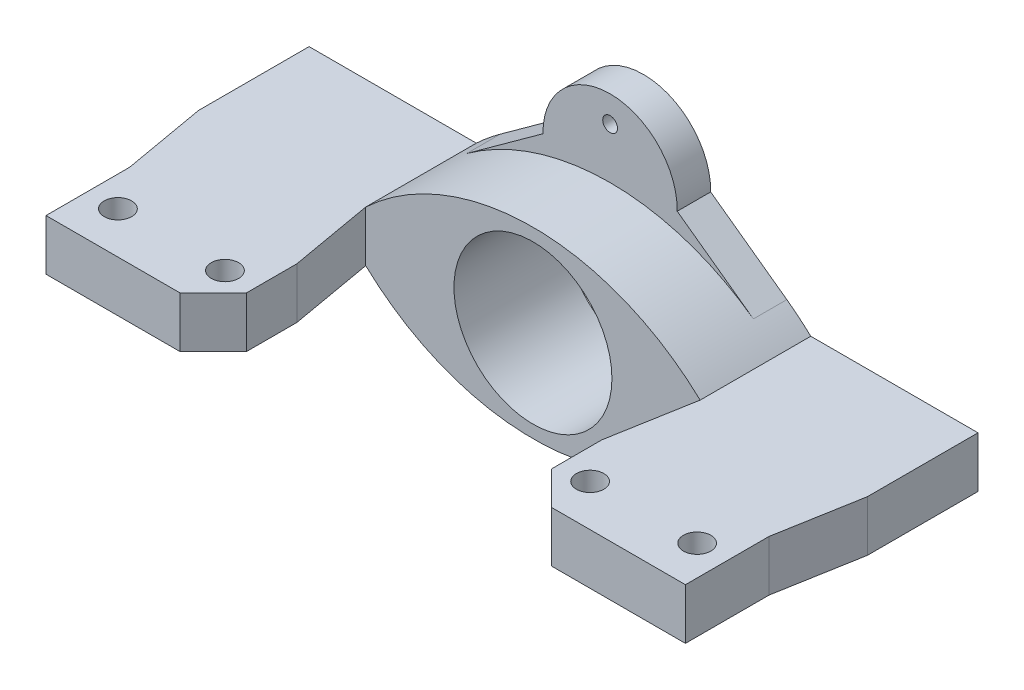
SolidWorks part; units mm, degrees
ref_plane "Front Plane" through (0, 0, 0) normal (0, 0, 1) x (1, 0, 0)
ref_plane "Top Plane" through (0, 0, 0) normal (0, 1, 0) x (1, 0, 0)
ref_plane "Right Plane" through (0, 0, 0) normal (1, 0, 0) x (0, 0, -1)
sketch "Sketch1" plane through (0, 0, 0) normal (0, 0, 1) x (1, 0, 0)
  line L1 (-25.7118, -19.05) -> (25.7118, -19.05)
  line L2 (-25.7118, -19.05) -> (-25.7118, 19.05)
  line L3 (-25.7118, 19.05) -> (25.7118, 19.05)
  line L4 (25.7118, -19.05) -> (25.7118, 19.05)
  line L5 (-25.7118, -19.05) -> (25.7118, 19.05) construction
  line L6 (-25.7118, 19.05) -> (25.7118, -19.05) construction
  line L7 (-63.5, -19.05) -> (63.5, -19.05)
  line L8 (-63.5, -19.05) -> (-63.5, 19.05)
  line L9 (-63.5, 19.05) -> (63.5, 19.05)
  line L10 (63.5, -19.05) -> (63.5, 19.05)
  line L11 (-63.5, -19.05) -> (63.5, 19.05) construction
  line L12 (-63.5, 19.05) -> (63.5, -19.05) construction
  circle A0 centre (0, 0) radius 15 construction
  circle A1 centre (0, 0) radius 15
  circle A2 centre (0, 0) radius 32 construction
  circle A3 centre (0, 0) radius 32
  dimension "D1" = 38.1
  dimension "D2" = 127
extrude "Boss-Extrude1" add sketch "Sketch1" against normal up to surface (21 mm away) contours A1 L3 L2 L1 | L2 A3 | A1 L1 L4 L3 | L4 A3 | A3 L9 L8 L7 | A3 L7 L10 L9
sketch "Sketch3" plane through (0, 0, -21) normal (0, 0, -1) x (-1, 0, 0)
  line L0 (0, 0) -> (0, -27) construction
  line L2 (-63.5, -19.05) -> (63.5, -19.05)
  line L3 (63.5, 19.05) -> (-63.5, 19.05)
  line L4 (-63.5, -19.05) -> (63.5, -19.05)
  line L5 (63.5, 19.05) -> (-63.5, 19.05)
  line L9 (63.5, -19.05) -> (63.5, 19.05)
  line L10 (63.5, -19.05) -> (63.5, 19.05)
  line L11 (-63.5, 19.05) -> (-63.5, -19.05)
  line L12 (-63.5, 19.05) -> (-63.5, -19.05)
  arc A0 (12.7437, -19.05) -> (-12.7437, -19.05) centre (0, -19.2546) cw
  circle A1 centre (0, 0) radius 32
  circle A6 centre (0, 0) radius 32
  dimension "D1" = 0
  dimension "D2" = 0
extrude "Boss-Extrude2" add sketch "Sketch3" against normal blind 6.35
sketch "Sketch4" plane through (0, 0, -14.65) normal (0, 0, 1) x (1, 0, 0)
  line L1 (12.7437, -19.05) -> (-12.7437, -19.05)
  line L2 (12.7437, -19.05) -> (-12.7437, -19.05)
  circle A0 centre (0, -27) radius 1.4 construction
  arc A1 (-12.7437, -19.05) -> (12.7437, -19.05) centre (0, -19.2546) ccw
  arc A2 (-12.7437, -19.05) -> (12.7437, -19.05) centre (0, -19.2546) ccw
  circle A3 centre (0, -27) radius 1.4
  dimension "D1" = 0
extrude "Cut-Extrude2" cut sketch "Sketch4" against normal blind 6.35 contours A3
ref_plane "Plane1" through (0, 0, 0) normal (0, 1, 0) x (1, 0, 0)
mirror "Mirror1" about plane through (0, 0, 0) normal (0, 1, 0) of "Boss-Extrude2", "Cut-Extrude2"
sketch "Sketch5" plane through (0, 0, 0) normal (0, 0, 1) x (1, 0, 0)
  line L0 (-63.5, 0) -> (0, 0) construction
  line L1 (-63.5, -4.826) -> (63.5, -4.826)
  line L2 (-63.5, -4.826) -> (-63.5, 4.826)
  line L3 (-63.5, 4.826) -> (63.5, 4.826)
  line L4 (-63.5, -19.05) -> (63.5, -19.05)
  line L5 (63.5, -19.05) -> (63.5, 19.05)
  line L6 (63.5, 19.05) -> (-63.5, 19.05)
  line L7 (-63.5, 19.05) -> (-63.5, -19.05)
  line L8 (-63.5, -19.05) -> (63.5, -19.05)
  line L9 (63.5, -19.05) -> (63.5, 19.05)
  line L10 (63.5, 19.05) -> (-63.5, 19.05)
  line L11 (-63.5, 19.05) -> (-63.5, -19.05)
  line L12 (63.5, -4.826) -> (63.5, 4.826)
  line L13 (-63.5, -4.826) -> (63.5, 4.826) construction
  line L14 (-63.5, 4.826) -> (63.5, -4.826) construction
  line L15 (0, 48.7566) -> (0, -50.4513) construction
  circle A0 centre (0, 0) radius 15 construction
  circle A1 centre (0, 0) radius 15
  arc A2 (31.75, 4.826) -> (-31.75, 4.826) centre (0, -28.9962) ccw
  arc A3 (31.75, -4.826) -> (-31.75, -4.826) centre (0, 28.9962) cw
  point P2 (0, 0)
  point P17 (-31.75, 0)
  circle M7 centre (0, 0) radius 15
  line M8 (-63.5, -19.05) -> (63.5, -19.05)
  line M9 (63.5, -19.05) -> (63.5, 19.05)
  line M10 (63.5, 19.05) -> (-63.5, 19.05)
  line M11 (-63.5, 19.05) -> (-63.5, -19.05)
  dimension "D2" = 9.652
  dimension "D1" = 0
extrude "Cut-Extrude6" cut sketch "Sketch5" against normal up to surface (14.65 mm away) contours A2 L3 M9 M10 M11 | L1 M11 M8 M9 M7
sketch "Sketch6" plane through (0, 0, -14.65) normal (0, 0, 1) x (1, 0, 0)
  line L6 (12.7437, -19.05) -> (63.5, -19.05)
  line L7 (63.5, -19.05) -> (63.5, -4.826)
  line L8 (63.5, -4.826) -> (31.75, -4.826)
  line L9 (-31.75, -4.826) -> (-63.5, -4.826)
  line L10 (-63.5, -4.826) -> (-63.5, -19.05)
  line L11 (-63.5, -19.05) -> (-12.7437, -19.05)
  line L12 (12.7437, -19.05) -> (63.5, -19.05)
  line L13 (63.5, -19.05) -> (63.5, -4.826)
  line L14 (63.5, -4.826) -> (31.75, -4.826)
  line L15 (-31.75, -4.826) -> (-63.5, -4.826)
  line L16 (-63.5, -4.826) -> (-63.5, -19.05)
  line L17 (-63.5, -19.05) -> (-12.7437, -19.05)
  line L18 (-12.7437, 19.05) -> (-63.5, 19.05)
  line L19 (-63.5, 19.05) -> (-63.5, 4.826)
  line L20 (-63.5, 4.826) -> (-31.75, 4.826)
  line L21 (31.75, 4.826) -> (63.5, 4.826)
  line L22 (63.5, 4.826) -> (63.5, 19.05)
  line L23 (63.5, 19.05) -> (12.7437, 19.05)
  line L24 (-12.7437, 19.05) -> (-63.5, 19.05)
  line L25 (-63.5, 19.05) -> (-63.5, 4.826)
  line L26 (-63.5, 4.826) -> (-31.75, 4.826)
  line L27 (31.75, 4.826) -> (63.5, 4.826)
  line L28 (63.5, 4.826) -> (63.5, 19.05)
  line L29 (63.5, 19.05) -> (12.7437, 19.05)
  line L30 (-12.7437, 19.05) -> (-27.2065, 8.5779)
  line L31 (12.7437, 19.05) -> (27.2065, 8.5779)
  line L32 (-69.4029, 0) -> (76.0293, 0) construction
  line L33 (12.7437, -19.05) -> (27.2065, -8.5779)
  line L34 (-12.7437, -19.05) -> (-27.2065, -8.5779)
  line L35 (12.7437, 19.05) -> (27.2065, 8.5779)
  arc A2 (-12.7437, -19.05) -> (12.7437, -19.05) centre (0, -19.2546) ccw
  arc A3 (-31.75, -4.826) -> (31.75, -4.826) centre (0, 28.9962) ccw
  arc A4 (-12.7437, -19.05) -> (12.7437, -19.05) centre (0, -19.2546) ccw
  arc A5 (-31.75, -4.826) -> (31.75, -4.826) centre (0, 28.9962) ccw
  arc A6 (12.7437, 19.05) -> (-12.7437, 19.05) centre (0, 19.2546) ccw
  arc A7 (31.75, 4.826) -> (-31.75, 4.826) centre (0, -28.9962) ccw
  arc A8 (12.7437, 19.05) -> (-12.7437, 19.05) centre (0, 19.2546) ccw
  arc A9 (31.75, 4.826) -> (-31.75, 4.826) centre (0, -28.9962) ccw
  dimension "D1" = 0
  dimension "D2" = 0
extrude "Cut-Extrude7" cut sketch "Sketch6" against normal through all
sketch "Sketch7" plane through (0, 4.826, 0) normal (0, 1, 0) x (1, 0, 0)
  line L0 (-57.785, 10.5) -> (-37.465, 10.5) construction
  line L1 (-47.625, 10.5) -> (-47.625, 16.5893) construction
  line L2 (0, 36.5321) -> (0, -15.9713) construction
  line L4 (-63.5, 21) -> (-63.5, 0)
  line L5 (-63.5, 0) -> (-31.75, 0)
  line L6 (-31.75, 0) -> (-31.75, 21)
  line L7 (-31.75, 21) -> (-63.5, 21)
  line L8 (-63.5, 21) -> (-63.5, 0)
  line L9 (-63.5, 0) -> (-31.75, 0)
  line L10 (-31.75, 0) -> (-31.75, 21)
  line L11 (-31.75, 21) -> (-63.5, 21)
  line L12 (31.75, 21) -> (31.75, 0)
  line L13 (31.75, 0) -> (63.5, 0)
  line L14 (63.5, 0) -> (63.5, 21)
  line L15 (63.5, 21) -> (31.75, 21)
  line L16 (31.75, 21) -> (31.75, 0)
  line L17 (31.75, 0) -> (63.5, 0)
  line L18 (63.5, 0) -> (63.5, 21)
  line L19 (63.5, 21) -> (31.75, 21)
  circle A0 centre (-57.785, 10.5) radius 2.6035
  circle A1 centre (-37.465, 10.5) radius 2.6035
  circle A2 centre (57.785, 10.5) radius 2.6035
  circle A3 centre (37.465, 10.5) radius 2.6035
  dimension "D3" = 5.207
  dimension "D4" = 20.32
  dimension "D1" = 0
  dimension "D2" = 0
extrude "Cut-Extrude8" cut sketch "Sketch7" against normal blind 22.86 contours A0 | A1 | A3 | A2
sketch "Sketch8" plane through (0, -4.826, 0) normal (0, -1, 0) x (1, 0, 0)
  line L0 (-63.5, 0) -> (-60.7008, 15.875)
  line L1 (-63.5, 0) -> (-31.75, 0)
  line L2 (-60.7008, 15.875) -> (-60.7008, 31.75)
  line L3 (-60.7008, 31.75) -> (-28.9508, 31.75)
  line L4 (-63.5, 0) -> (-63.5, -21)
  line L5 (-63.5, -21) -> (-31.75, -21)
  line L6 (-31.75, -21) -> (-31.75, 0)
  line L7 (-31.75, 0) -> (-63.5, 0)
  line L8 (-63.5, 0) -> (-63.5, -21)
  line L9 (-63.5, -21) -> (-31.75, -21)
  line L10 (-31.75, -21) -> (-31.75, 0)
  line L11 (-31.75, 0) -> (-63.5, 0)
  line L12 (-28.9508, 31.75) -> (-28.9508, 15.875)
  line L13 (-28.9508, 15.875) -> (-31.75, 0)
  line L14 (0, 0) -> (0, 19.7976) construction
  line L15 (31.75, 0) -> (-31.75, 0) construction
  line L16 (-54.9858, 23.8125) -> (-34.6658, 23.8125) construction
  line L17 (-44.8258, 23.8125) -> (-44.8258, 29.1461) construction
  line L18 (-60.7008, 15.875) -> (-28.9508, 15.875)
  line L19 (63.5, 0) -> (31.75, 0)
  line L20 (44.8258, 23.8125) -> (44.8258, 29.1461) construction
  line L21 (54.9858, 23.8125) -> (34.6658, 23.8125) construction
  line L22 (60.7008, 15.875) -> (28.9508, 15.875)
  line L23 (28.9508, 15.875) -> (31.75, 0)
  line L24 (28.9508, 31.75) -> (28.9508, 15.875)
  line L25 (60.7008, 31.75) -> (28.9508, 31.75)
  line L26 (60.7008, 15.875) -> (60.7008, 31.75)
  line L27 (63.5, 0) -> (60.7008, 15.875)
  circle A0 centre (-54.9858, 23.8125) radius 2.6035
  circle A1 centre (-34.6658, 23.8125) radius 2.6035
  circle A2 centre (-57.785, -10.5) radius 2.6035 construction
  circle A3 centre (34.6658, 23.8125) radius 2.6035
  circle A4 centre (54.9858, 23.8125) radius 2.6035
  line M16 (-31.75, 0) -> (-63.5, 0)
  dimension "D2" = 31.75
  dimension "D3" = 15.875
  dimension "D4" = 80
  dimension "D5" = 20.32
  dimension "D1" = 0
extrude "Boss-Extrude3" add sketch "Sketch8" against normal up to surface (9.652 mm away) contours L19 L27 L22 L23 | L22 L26 L25 L24 A3 A4 | L2 L18 L12 L3 A1 A0 | L18 L0 L13 M16 up to face at (57.785, 4.826, -7.8965)
chamfer "Chamfer1" distance 6.35 angle 45 2 edges at (28.9508, 0, 31.75) (-28.9508, 0, 31.75)
sketch "Sketch9" plane through (0, -4.826, 0) normal (0, -1, 0) x (1, 0, 0)
  line L1 (-60.7008, -3.5963) -> (-34.0194, -3.5963)
  line L2 (-60.7008, -3.5963) -> (-60.7008, -15.4827)
  line L3 (-60.7008, -15.4827) -> (-34.0194, -15.4827)
  line L4 (-34.0194, -3.5963) -> (-34.0194, -15.4827)
  line L5 (34.2163, -3.5963) -> (61.2099, -3.5963)
  line L6 (34.2163, -3.5963) -> (34.2163, -15.4827)
  line L7 (34.2163, -15.4827) -> (61.2099, -15.4827)
  line L8 (61.2099, -3.5963) -> (61.2099, -15.4827)
  line L9 (-28.9508, 15.875) -> (-28.9508, 25.4)
  line L10 (-28.9508, 25.4) -> (-35.3008, 31.75)
  line L11 (-35.3008, 31.75) -> (-60.7008, 31.75)
  line L12 (-60.7008, 31.75) -> (-60.7008, 15.875)
  line L13 (-60.7008, 15.875) -> (-63.5, 0)
  line L14 (-63.5, 0) -> (-63.5, -21)
  line L15 (-63.5, -21) -> (-31.75, -21)
  line L16 (-31.75, -21) -> (-31.75, 0)
  line L17 (-31.75, 0) -> (-28.9508, 15.875)
  line L18 (-28.9508, 15.875) -> (-28.9508, 25.4)
  line L19 (-28.9508, 25.4) -> (-35.3008, 31.75)
  line L20 (-35.3008, 31.75) -> (-60.7008, 31.75)
  line L21 (-60.7008, 31.75) -> (-60.7008, 15.875)
  line L22 (-60.7008, 15.875) -> (-63.5, 0)
  line L23 (-63.5, 0) -> (-63.5, -21)
  line L24 (-63.5, -21) -> (-31.75, -21)
  line L25 (-31.75, -21) -> (-31.75, 0)
  line L26 (-31.75, 0) -> (-28.9508, 15.875)
  circle M10 centre (-37.465, -10.5) radius 2.6035
  circle M11 centre (-57.785, -10.5) radius 2.6035
  dimension "D1" = 0
extrude "Boss-Extrude4" add sketch "Sketch9" against normal up to surface (9.652 mm away) contours L4 L1 L2 L3 M11 M10 | M11 | M10 | L8 L5 L6 L7 up to face at (-37.465, 4.826, -7.8965)
